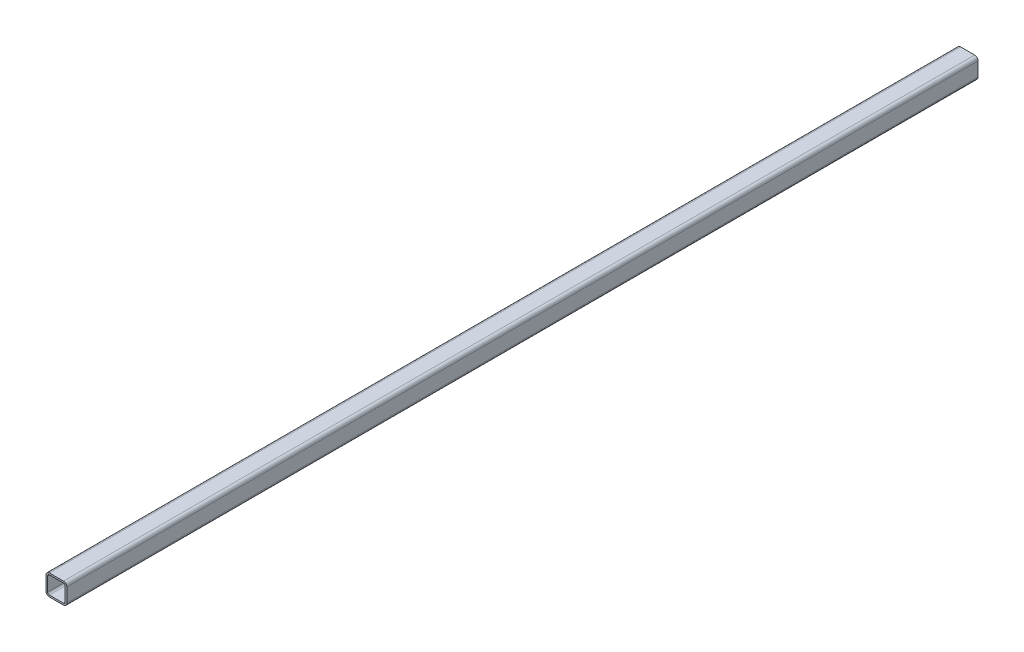
from build123d import *

# Parameters (mm, degrees)
BOSS_EXTRUDE1_DEPTH = 1094


with BuildPart() as part:
    # Sketch1 → Boss-Extrude1 (new body)
    with BuildSketch(Plane.XY):
        with BuildLine():
            Line((-8.5, -12.5), (8.5, -12.5))
            ThreePointArc((8.5, -12.5), (11.328427125, -11.328427125), (12.5, -8.5))
            Line((12.5, -8.5), (12.5, 8.5))
            ThreePointArc((12.5, 8.5), (11.328427125, 11.328427125), (8.5, 12.5))
            Line((8.5, 12.5), (-8.5, 12.5))
            ThreePointArc((-8.5, 12.5), (-11.328427125, 11.328427125), (-12.5, 8.5))
            Line((-12.5, 8.5), (-12.5, -8.5))
            ThreePointArc((-12.5, -8.5), (-11.328427125, -11.328427125), (-8.5, -12.5))
        make_face()
        with BuildLine():
            Line((-8.5, -10.5), (8.5, -10.5))
            ThreePointArc((8.5, -10.5), (9.914213562, -9.914213562), (10.5, -8.5))
            Line((10.5, -8.5), (10.5, 8.5))
            ThreePointArc((10.5, 8.5), (9.914213562, 9.914213562), (8.5, 10.5))
            Line((8.5, 10.5), (-8.5, 10.5))
            ThreePointArc((-8.5, 10.5), (-9.914213562, 9.914213562), (-10.5, 8.5))
            Line((-10.5, 8.5), (-10.5, -8.5))
            ThreePointArc((-10.5, -8.5), (-9.914213562, -9.914213562), (-8.5, -10.5))
        make_face(mode=Mode.SUBTRACT)
    extrude(amount=BOSS_EXTRUDE1_DEPTH)


solid = part.part
